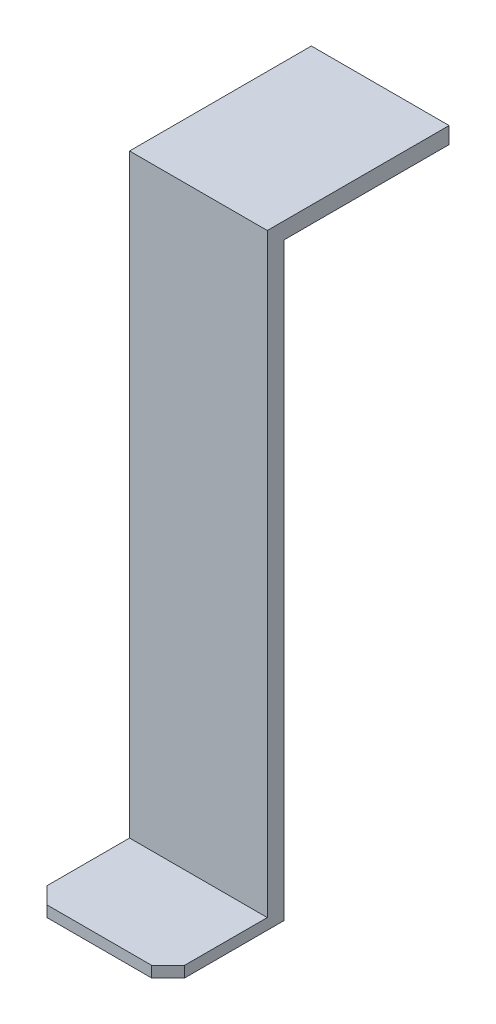
SolidWorks part; units mm, degrees
ref_plane "前视基准面" through (0, 0, 0) normal (0, 0, 1) x (1, 0, 0)
ref_plane "上视基准面" through (0, 0, 0) normal (0, 1, 0) x (1, 0, 0)
ref_plane "右视基准面" through (0, 0, 0) normal (1, 0, 0) x (0, 0, -1)
sketch "草图1" plane through (0, 0, 0) normal (0, 0, 1) x (1, 0, 0)
  line L1 (-12.5, -55) -> (12.5, -55)
  line L2 (-12.5, -55) -> (-12.5, 55)
  line L3 (-12.5, 55) -> (12.5, 55)
  line L4 (12.5, -55) -> (12.5, 55)
  line L5 (-12.5, -55) -> (12.5, 55) construction
  line L6 (-12.5, 55) -> (12.5, -55) construction
  point P0 (0, 0)
  dimension "D1" = 25
  dimension "D2" = 110
extrude "凸台-拉伸1" add sketch "草图1" along normal blind 3
sketch "草图3" plane through (0, 0, 3) normal (0, 0, 1) x (1, 0, 0)
  line L0 (12.5, -55) -> (12.5, 55) construction
  line L1 (-12.5, -55) -> (12.5, -55)
  line L2 (-12.5, -55) -> (-12.5, -53)
  line L3 (-12.5, -53) -> (12.5, -53)
  line L4 (12.5, -55) -> (12.5, -53)
  dimension "D1" = 2
extrude "凸台-拉伸2" add sketch "草图3" along normal blind 18
sketch "草图4" plane through (0, 0, 0) normal (0, 0, -1) x (-1, 0, 0)
  line L0 (12.5, 55) -> (12.5, -55) construction
  line L1 (-12.5, 55) -> (12.5, 55)
  line L2 (-12.5, 55) -> (-12.5, 52)
  line L3 (-12.5, 52) -> (12.5, 52)
  line L4 (12.5, 55) -> (12.5, 52)
  dimension "D1" = 3
extrude "凸台-拉伸3" add sketch "草图4" along normal blind 30
chamfer "倒角1" distance 3 angle 45 2 edges at (12.5, -54, 21) (-12.5, -54, 21)
